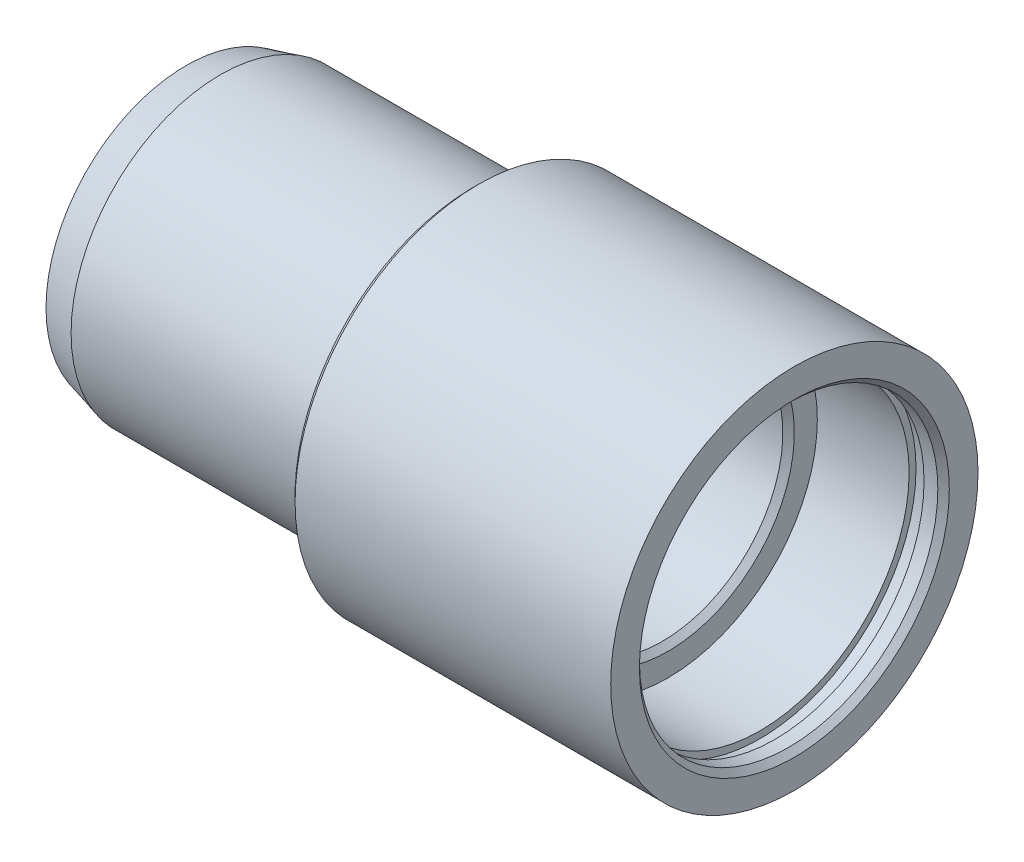
SolidWorks part; units mm, degrees
ref_plane "前视基准面" through (0, 0, 0) normal (0, 0, 1) x (1, 0, 0)
ref_plane "上视基准面" through (0, 0, 0) normal (0, 1, 0) x (1, 0, 0)
ref_plane "右视基准面" through (0, 0, 0) normal (1, 0, 0) x (0, 0, -1)
sketch "草图1" plane through (0, 0, 0) normal (0, 1, 0) x (1, 0, 0)
  line L0 (0, 0) -> (46.9495, 0) construction
  line L1 (-28.6143, 10.5) -> (13.3857, 10.5)
  line L2 (13.3857, 10.5) -> (13.3857, 13)
  line L3 (13.3857, 13) -> (21.3857, 13)
  line L4 (21.3857, 13) -> (21.3857, 13.6)
  line L5 (21.3857, 13.6) -> (22.6857, 13.6)
  line L6 (22.6857, 13.6) -> (22.6857, 13)
  line L7 (22.6857, 13) -> (24.3857, 13)
  line L8 (24.3857, 13) -> (24.3857, 16)
  line L9 (24.3857, 16) -> (-3.6143, 16)
  line L10 (-3.6143, 16) -> (-3.6143, 13)
  line L11 (-3.6143, 13) -> (-25.6286, 13)
  line L12 (-25.6286, 13) -> (-28.6143, 12.2)
  line L13 (-28.6143, 12.2) -> (-28.6143, 10.5)
  dimension "D1" = 10.5
  dimension "D2" = 42
  dimension "D3" = 13
  dimension "D4" = 8
  dimension "D5" = 0.6
  dimension "D6" = 0.6
  dimension "D7" = 1.3
  dimension "D8" = 1.7
  dimension "D9" = 3
  dimension "D10" = 28
  dimension "D11" = 3
  dimension "D12" = 1.7
revolve "旋转1" add sketch "草图1" angle 360 about L0
chamfer "倒角1" distance 0.5 angle 45 4 edges at (-3.6143, 0, 16) (24.3857, 0, 13) (13.3857, 0, 10.5) (-28.6143, 0, 10.5)
